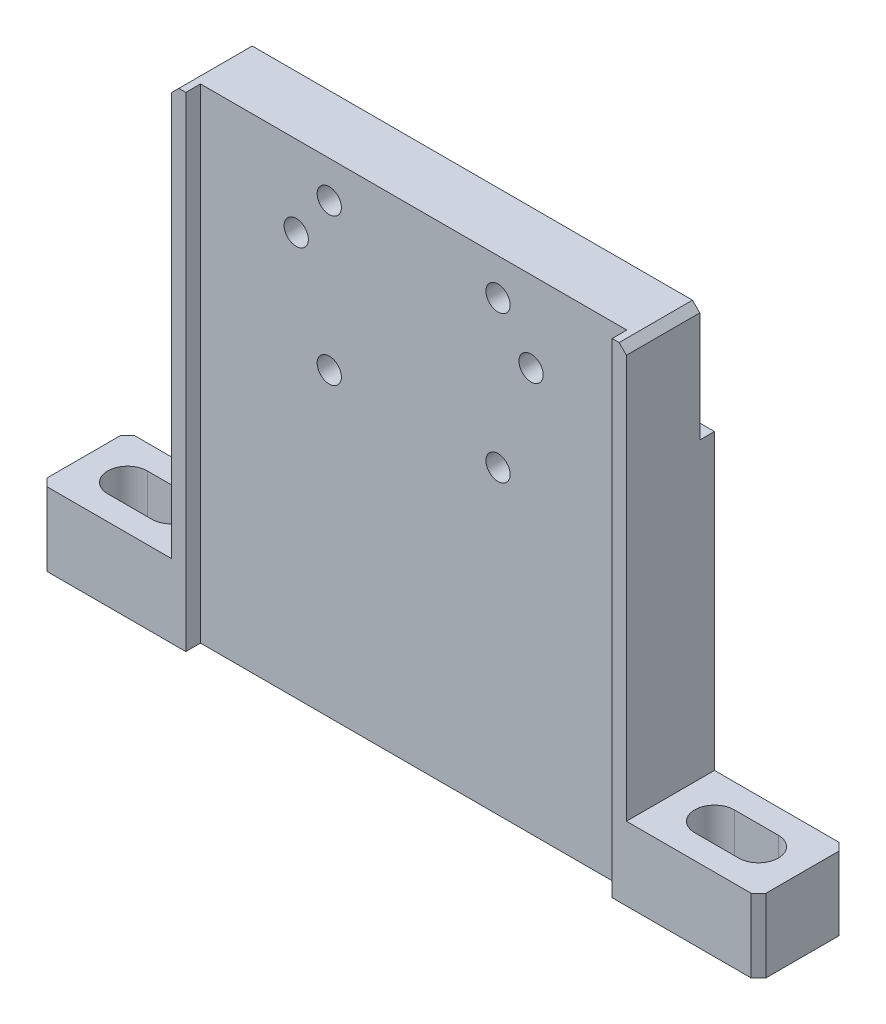
SolidWorks part; units mm, degrees
ref_plane "前视基准面" through (0, 0, 0) normal (0, 0, 1) x (1, 0, 0)
ref_plane "上视基准面" through (0, 0, 0) normal (0, 1, 0) x (1, 0, 0)
ref_plane "右视基准面" through (0, 0, 0) normal (1, 0, 0) x (0, 0, -1)
sketch "草图1" plane through (0, 0, 0) normal (0, 0, 1) x (1, 0, 0)
  line L1 (-31, 33) -> (31, 33)
  line L2 (-31, 33) -> (-31, -33)
  line L3 (-31, -33) -> (31, -33)
  line L4 (31, 33) -> (31, -33)
  line L5 (-31, 33) -> (31, -33) construction
  line L6 (-31, -33) -> (31, 33) construction
  point P0 (0, 0)
  dimension "D1" = 62
  dimension "D2" = 66
extrude "凸台-拉伸1" add sketch "草图1" along normal mid plane 12
sketch "草图2" plane through (0, -33, 0) normal (0, -1, 0) x (1, 0, 0)
  line L0 (-31, 6) -> (31, 6) construction
  line L1 (-41, 6) -> (41, 6)
  line L2 (-41, 6) -> (-41, -6)
  line L3 (-41, -6) -> (41, -6)
  line L4 (41, 6) -> (41, -6)
  line L5 (-41, 6) -> (41, -6) construction
  line L6 (-41, -6) -> (41, 6) construction
  point P0 (0, 0)
  dimension "D1" = 82
extrude "凸台-拉伸2" [suppressed] add sketch "草图2" against normal blind 10
sketch "草图3" plane through (0, 0, 6) normal (0, 0, 1) x (1, 0, 0)
  line L1 (-29.05, 56.8456) -> (29.05, 56.8456)
  line L2 (-29.05, 56.8456) -> (-29.05, -56.8456)
  line L3 (-29.05, -56.8456) -> (29.05, -56.8456)
  line L4 (29.05, 56.8456) -> (29.05, -56.8456)
  line L5 (-29.05, 56.8456) -> (29.05, -56.8456) construction
  line L6 (-29.05, -56.8456) -> (29.05, 56.8456) construction
  point P0 (0, 0)
  dimension "D1" = 58.1
extrude "切除-拉伸1" cut sketch "草图3" against normal blind 2
hole_wizard "Ø5.5 (5.5) 直径孔1" positions "草图5" profile "草图4" hole size "Ø5.5" standard "GB"
sketch "草图5" [suppressed] plane through (0, -29, 0) normal (0, 1, 0) x (1, 0, 0)
  line L0 (-36, 0) -> (36, 0) construction
  point P0 (-36, 0)
  point P2 (36, 0)
  dimension "D1" = 72
sketch "草图4" plane through (-36, -29, 0) normal (1, 0, 0) x (0, 0, 1)
  line L0 (0, 0) -> (0, 10)
  line L1 (0, 10) -> (2.75, 10)
  line L2 (2.75, 10) -> (2.75, 0)
  line L5 (2.75, 0) -> (0, 0)
  line L11 (0, -6.35) -> (0, 107.95) construction
  dimension "通孔孔直径" = 5.5
  dimension "通孔孔深度" = 10
hole_wizard "M5 螺纹孔1" positions "草图8" profile "草图6" tap size "M5" standard "GB"
sketch "草图8" plane through (0, -38, 0) normal (0, -1, 0) x (-1, 0, 0)
  line L0 (20, 1) -> (-20, 1) construction
  line L3 (31, 6) -> (-31, 6) construction
  line L4 (0, 0) -> (0, 1) construction
  point P0 (20, 1)
  point P2 (-20, 1)
  dimension "D1" = 5
  dimension "D2" = 40
sketch "草图6" plane through (-20, -38, -1) normal (1, 0, 0) x (0, 0, -1)
  line L0 (0, 0) -> (0, 20.2618)
  line L1 (0, 20.2618) -> (2.1, 19)
  line L2 (2.1, 19) -> (2.1, 0)
  line L5 (2.1, 0) -> (0, 0)
  line L10 (0, 20.2618) -> (-2.1, 19) construction
  line L11 (0, -6.35) -> (0, 107.95) construction
  dimension "螺纹孔钻头直径" = 4.2
  dimension "螺纹孔钻头深度" = 19
  dimension "导头角度" = 118
cosmetic thread "孔螺蚊线1" [suppressed] parameters "D1"=15, "D2"=5
cosmetic thread "孔螺蚊线2" [suppressed] parameters "D1"=15, "D2"=5
hole_wizard "M4 螺纹孔1" positions "草图10" profile "草图9" tap size "M4" standard "GB" end condition through all
sketch "草图10" plane through (0, 0, 4) normal (0, 0, 1) x (1, 0, 0)
  line L0 (-11.5, 28) -> (11.5, 28) construction
  line L3 (0, 33) -> (0, 28) construction
  line L4 (29.05, 33) -> (-29.05, 33) construction
  point P0 (-11.5, 28)
  point P2 (11.5, 28)
  point P4 (-11.5, 8)
  point P6 (11.5, 8)
  dimension "D1" = 5
  dimension "D2" = 23
  dimension "D3" = 20
sketch "草图9" plane through (-11.5, 28, 4) normal (1, 0, 0) x (0, -1, 0)
  line L0 (0, 0) -> (0, 10)
  line L1 (0, 10) -> (1.65, 10)
  line L2 (1.65, 10) -> (1.65, 0)
  line L5 (1.65, 0) -> (0, 0)
  line L11 (0, -6.35) -> (0, 107.95) construction
  dimension "通孔螺纹孔钻头直径" = 3.3
  dimension "通孔螺纹孔钻头深度" = 10
cosmetic thread "孔螺蚊线3" parameters "D2"=4
cosmetic thread "孔螺蚊线4" parameters "D2"=4
cosmetic thread "孔螺蚊线5" parameters "D2"=4
cosmetic thread "孔螺蚊线6" parameters "D2"=4
hole_wizard "M4 螺纹孔2" positions "草图13" profile "草图12" tap size "M4" standard "GB" end condition through all
sketch "草图13" plane through (0, 0, -6) normal (0, 0, -1) x (-1, 0, 0)
  line L0 (-16, 22) -> (16, 22) construction
  line L3 (0, 22) -> (0, 0) construction
  line L6 (-31, 33) -> (31, 33) construction
  point P0 (-16, 22)
  point P2 (16, 22)
  dimension "D1" = 11
  dimension "D2" = 32
sketch "草图12" plane through (16, 22, -6) normal (1, 0, 0) x (0, 1, 0)
  line L0 (0, 0) -> (0, 12)
  line L1 (0, 12) -> (1.65, 12)
  line L2 (1.65, 12) -> (1.65, 0)
  line L5 (1.65, 0) -> (0, 0)
  line L11 (0, -6.35) -> (0, 107.95) construction
  dimension "通孔螺纹孔钻头直径" = 3.3
  dimension "通孔螺纹孔钻头深度" = 12
cosmetic thread "孔螺蚊线7" parameters "D2"=4
cosmetic thread "孔螺蚊线8" parameters "D2"=4
sketch "草图14" plane through (0, -33, 0) normal (0, -1, 0) x (1, 0, 0)
  line L1 (-49, 6) -> (49, 6)
  line L2 (-49, 6) -> (-49, -6)
  line L3 (-49, -6) -> (49, -6)
  line L4 (49, 6) -> (49, -6)
  line L5 (-49, 6) -> (49, -6) construction
  line L6 (-49, -6) -> (49, 6) construction
  point P0 (0, 0)
  dimension "D1" = 98
  dimension "D2" = 12
extrude "凸台-拉伸3" add sketch "草图14" against normal blind 10
sketch "草图15" plane through (0, -23, 0) normal (0, 1, 0) x (1, 0, 0)
  line L0 (-43, 0) -> (-37, 0) construction
  line L1 (-43, 2.7) -> (-37, 2.7)
  line L2 (-43, -2.7) -> (-37, -2.7)
  arc A0 (-43, 2.7) -> (-43, -2.7) centre (-43, 0) ccw
  arc A1 (-37, -2.7) -> (-37, 2.7) centre (-37, 0) ccw
  point P2 (-40, 0)
  dimension "D1" = 40
  dimension "D2" = 6
  dimension "D3" = 5.4
extrude "切除-拉伸2" cut sketch "草图15" against normal through all
mirror "镜向1" about plane through (0, 0, 0) normal (1, 0, 0) of "切除-拉伸2"
sketch "草图16" plane through (0, 0, 6) normal (0, 0, 1) x (1, 0, 0)
  line L0 (29.05, -23) -> (29.05, 33) construction
  line L1 (29.05, -59.7808) -> (-29.05, -59.7808)
  line L2 (29.05, -59.7808) -> (29.05, -18.495)
  line L3 (29.05, -18.495) -> (-29.05, -18.495)
  line L4 (-29.05, -59.7808) -> (-29.05, -18.495)
  line L5 (29.05, -59.7808) -> (-29.05, -18.495) construction
  line L6 (29.05, -18.495) -> (-29.05, -59.7808) construction
  point P0 (0, -39.1379)
extrude "切除-拉伸3" cut sketch "草图16" against normal blind 2
sketch "草图17" plane through (0, 0, -6) normal (0, 0, -1) x (-1, 0, 0)
  line L0 (-31, 33) -> (31, 33) construction
  line L1 (-71.9013, 70.479) -> (54.3341, 70.479)
  line L2 (-71.9013, 70.479) -> (-71.9013, 17)
  line L3 (-71.9013, 17) -> (54.3341, 17)
  line L4 (54.3341, 70.479) -> (54.3341, 17)
  line L5 (-71.9013, 70.479) -> (54.3341, 17) construction
  line L6 (-71.9013, 17) -> (54.3341, 70.479) construction
  point P0 (-8.7836, 43.7395)
  dimension "D1" = 16
extrude "切除-拉伸4" cut sketch "草图17" against normal blind 2
chamfer "倒角1" distance 1 angle 45 4 edges at (-49, -28, -6) (-49, -28, 6) (49, -28, -6) (49, -28, 6)
chamfer "倒角2" distance 1 angle 45 2 edges at (-31, 33, 1) (31, 33, 1)
